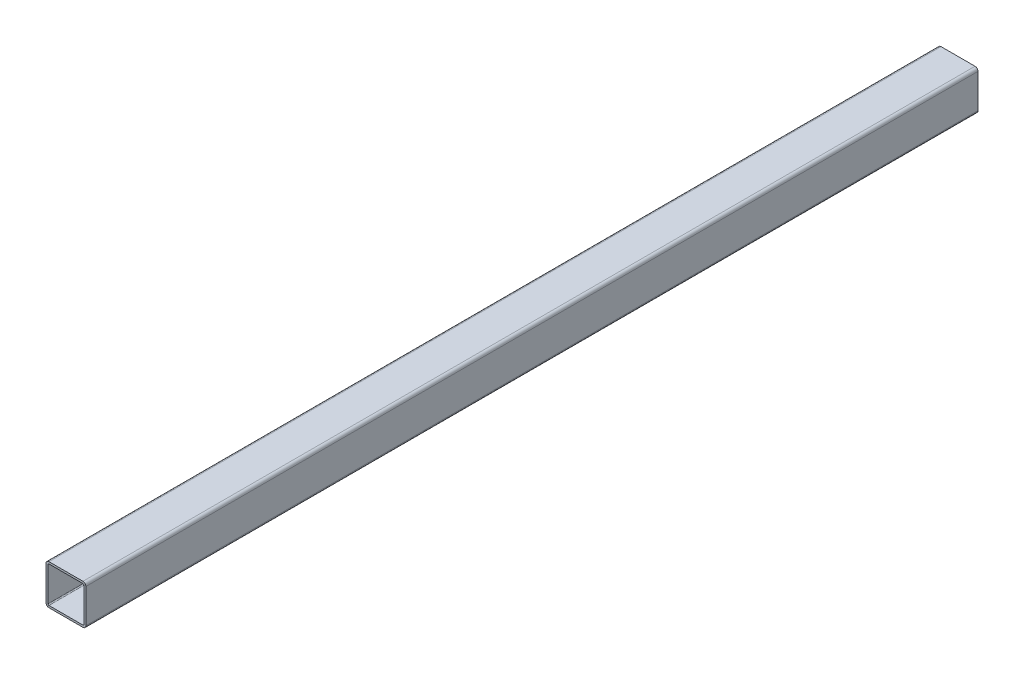
SolidWorks part; units mm, degrees
ref_plane "Front Plane" through (0, 0, 0) normal (0, 0, 1) x (1, 0, 0)
ref_plane "Top Plane" through (0, 0, 0) normal (0, 1, 0) x (1, 0, 0)
ref_plane "Right Plane" through (0, 0, 0) normal (1, 0, 0) x (0, 0, -1)
sketch "Sketch 1" plane through (0, 0, 0) normal (0, 0, 1) x (1, 0, 0)
  line L0 (0, 96.8978) -> (0, -107.4818) construction
  line L1 (-129.1971, 0) -> (137.9562, 0) construction
  line L2 (0, 40.5) -> (-34.5, 40.5)
  line L3 (-40.5, 34.5) -> (-40.5, 0)
  line L4 (0, 36.5) -> (-34.5, 36.5)
  line L5 (-36.5, 34.5) -> (-36.5, 0)
  line L6 (-36.5, -34.5) -> (-36.5, 0)
  line L7 (34.5, -36.5) -> (-34.5, -36.5)
  line L8 (-40.5, -34.5) -> (-40.5, 0)
  line L9 (34.5, -40.5) -> (-34.5, -40.5)
  line L10 (40.5, -34.5) -> (40.5, 0)
  line L11 (36.5, -34.5) -> (36.5, 0)
  line L12 (36.5, 34.5) -> (36.5, 0)
  line L13 (0, 36.5) -> (34.5, 36.5)
  line L14 (40.5, 34.5) -> (40.5, 0)
  line L15 (0, 40.5) -> (34.5, 40.5)
  arc A0 (-34.5, 40.5) -> (-40.5, 34.5) centre (-34.5, 34.5) ccw
  arc A1 (-34.5, 36.5) -> (-36.5, 34.5) centre (-34.5, 34.5) ccw
  arc A2 (-34.5, -36.5) -> (-36.5, -34.5) centre (-34.5, -34.5) cw
  arc A3 (-34.5, -40.5) -> (-40.5, -34.5) centre (-34.5, -34.5) cw
  arc A4 (34.5, -40.5) -> (40.5, -34.5) centre (34.5, -34.5) ccw
  arc A5 (34.5, -36.5) -> (36.5, -34.5) centre (34.5, -34.5) ccw
  arc A6 (34.5, 36.5) -> (36.5, 34.5) centre (34.5, 34.5) cw
  arc A7 (34.5, 40.5) -> (40.5, 34.5) centre (34.5, 34.5) cw
  point P34 (0, -40.5)
  point P35 (0, -36.5)
  dimension "D3" = 6
  dimension "D1" = 81
  dimension "D2" = 81
  dimension "D4" = 4
extrude "Boss-Extrude 1" add sketch "Sketch 1" along normal mid plane 1811
